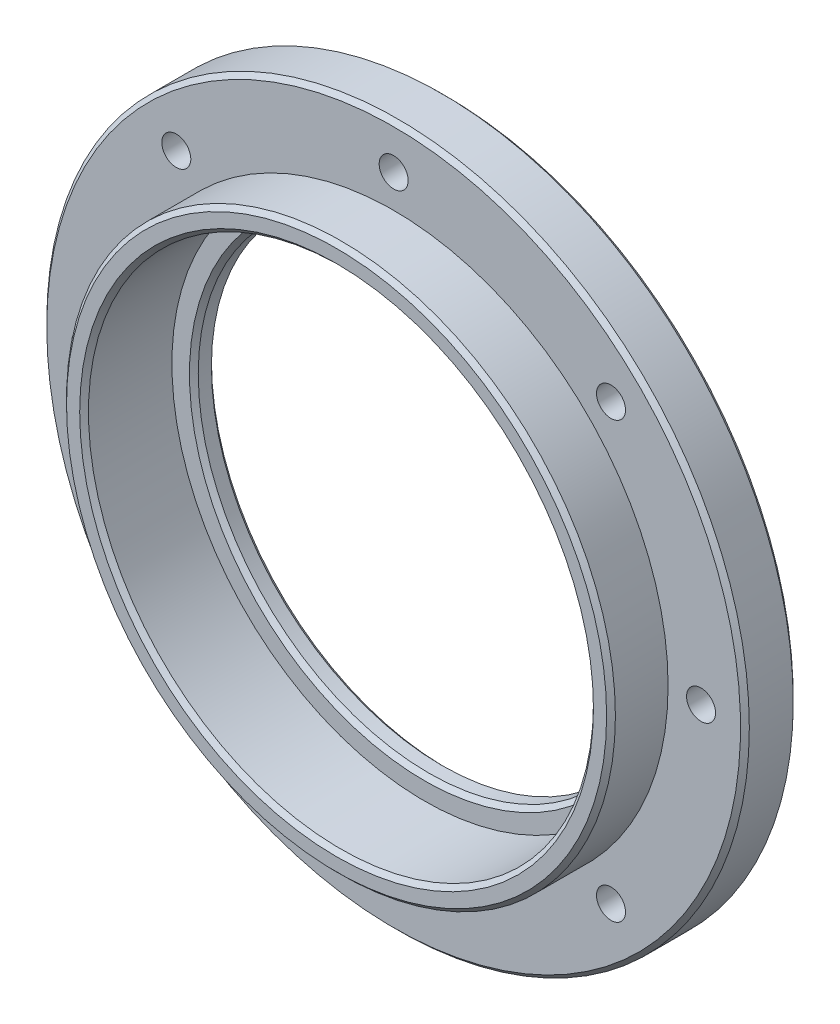
from build123d import *

# Parameters (mm, degrees)
SKETCH1_R           = 62.5
SKETCH1_R_2         = 57.5
BOSS_EXTRUDE1_DEPTH = 13
SKETCH2_R           = 80
SKETCH2_R_2         = 52.5
BOSS_EXTRUDE2_DEPTH = 12
CUT_EXTRUDE1_START  = -7
SKETCH3_R           = 57.5
CUT_EXTRUDE1_DEPTH  = 7
CIRPATTERN1_COUNT   = 8
CHAMFER1_SIZE       = 1


with BuildPart() as part:
    # Sketch1 → Boss-Extrude1 (new body)
    with BuildSketch(Plane.XY):
        Circle(SKETCH1_R)
        Circle(SKETCH1_R_2, mode=Mode.SUBTRACT)
    extrude(amount=BOSS_EXTRUDE1_DEPTH)

    # Sketch2 → Boss-Extrude2 (add)
    with BuildSketch(Plane(origin=(0, 0, 0), x_dir=(-1, 0, 0), z_dir=(0, 0, -1))):
        Circle(SKETCH2_R)
        Circle(SKETCH2_R_2, mode=Mode.SUBTRACT)
    extrude(amount=BOSS_EXTRUDE2_DEPTH)

    # Sketch3 → Cut-Extrude1 (cut)
    with BuildSketch(Plane.XY.offset(CUT_EXTRUDE1_START)):
        Circle(SKETCH3_R)
    extrude(amount=CUT_EXTRUDE1_DEPTH, mode=Mode.SUBTRACT)

    # Sketch5 → Hole size (%based on) socket head cap screw type1 (revolve, cut)
    with BuildSketch(Plane(origin=(-70, 0, -12), x_dir=(0, 1, 0), z_dir=(1, 0, 0))):
        Polygon((0, 0), (0, 26.482840043), (3.3, 24.5), (3.3, 6.8), (5.5, 6.8), (5.5, 0), align=None)
    hole_size_based_on_socket_head_cap_scr = revolve(axis=Axis((-70, 0, -18.35), (0, 0, 1)), mode=Mode.SUBTRACT)

    # CirPattern1: Hole size (%based on) socket head cap screw type1 ×8 about axis
    cirpattern1_axis = Axis((0, 0, 0), (0, 0, 1))
    for i in range(1, CIRPATTERN1_COUNT):
        add(hole_size_based_on_socket_head_cap_scr.rotate(cirpattern1_axis, i * 360 / CIRPATTERN1_COUNT), mode=Mode.SUBTRACT)

    # Chamfer1
    chamfer1_edges = [part.edges().sort_by_distance(p)[0] for p in [
        (80, 0, -12),
        (80, 0, 0),
        (52.5, 0, -12),
        (52.5, 0, -7),
        (-62.5, 0, 13),
        (-57.5, 0, 13),
    ]]
    chamfer(chamfer1_edges, length=CHAMFER1_SIZE)


solid = part.part
